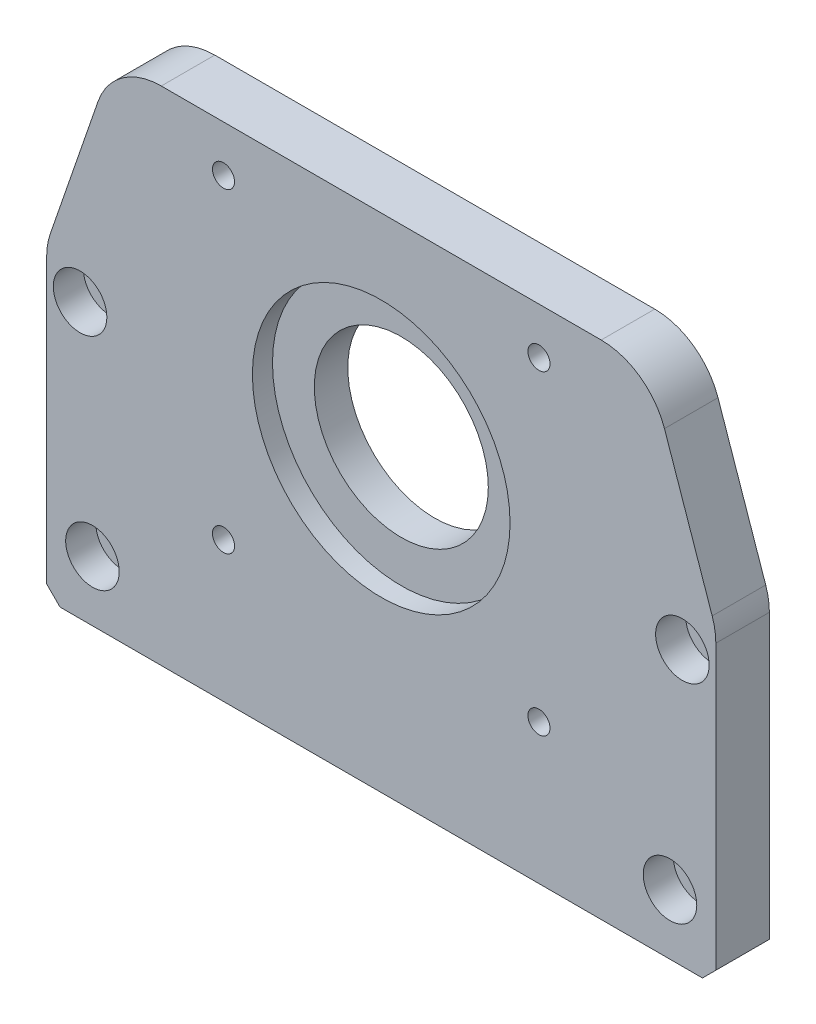
SolidWorks part; units mm, degrees
material "6061铝"
ref_plane "前视基准面" through (0, 0, 0) normal (0, 0, 1) x (1, 0, 0)
ref_plane "上视基准面" through (0, 0, 0) normal (0, 1, 0) x (1, 0, 0)
ref_plane "右视基准面" through (0, 0, 0) normal (1, 0, 0) x (0, 0, -1)
sketch "草图1" plane through (0, 0, 0) normal (0, 0, 1) x (1, 0, 0)
  line L1 (-50, -37.5) -> (50, -37.5)
  line L2 (-50, -37.5) -> (-50, 37.5)
  line L3 (-50, 37.5) -> (50, 37.5)
  line L4 (50, -37.5) -> (50, 37.5)
  line L5 (-50, -37.5) -> (50, 37.5) construction
  line L6 (-50, 37.5) -> (50, -37.5) construction
  point P0 (0, 0)
  dimension "D1" = 100
  dimension "D2" = 75
extrude "凸台-拉伸1" add sketch "草图1" along normal blind 8
sketch "草图3" plane through (0, 0, 0) normal (0, 0, -1) x (-1, 0, 0)
  line L0 (-50, 8.5) -> (-40, 37.5)
  line L1 (-50, -37.5) -> (-50, 37.5) construction
  line L2 (-50, 37.5) -> (50, 37.5) construction
  line L3 (-40, 37.5) -> (-50, 37.5)
  line L4 (-50, 37.5) -> (-50, 8.5)
  line L5 (50, -37.5) -> (-50, -37.5) construction
  line L6 (0, 37.5) -> (0, 59.5078) construction
  line L7 (50, 37.5) -> (50, 8.5)
  line L8 (40, 37.5) -> (50, 37.5)
  line L9 (50, 8.5) -> (40, 37.5)
  dimension "D1" = 46
  dimension "D2" = 10
extrude "切除-拉伸1" cut sketch "草图3" against normal blind 10
fillet "圆角1" radius 10 4 edges at (-50, 8.5, 4) (-40, 37.5, 4) (40, 37.5, 4) (50, 8.5, 4)
chamfer "倒角2" distance 2 angle 45 2 edges at (-50, -37.5, 4) (50, -37.5, 4)
sketch "草图6" plane through (0, 0, 8) normal (0, 0, 1) x (1, 0, 0)
  line L0 (-48, -37.5) -> (48, -37.5) construction
  line L1 (-50, 6.8243) -> (-50, -35.5) construction
  circle A0 centre (0, 7) radius 19.25
  dimension "D1" = 38.5
  dimension "D2" = 44.5
  dimension "D3" = 50
extrude "切除-拉伸2" cut sketch "草图6" against normal blind 3
sketch "草图7" plane through (0, 0, 5) normal (0, 0, 1) x (1, 0, 0)
  circle A0 centre (0, 7) radius 13
  dimension "D1" = 26
extrude "切除-拉伸3" cut sketch "草图7" against normal through all
hole_wizard "打孔尺寸(%根据)内六角圆柱头螺钉的类型1" positions "草图8" profile "草图9" counterbore size "M4" standard "GB" end condition through all
sketch "草图8" plane through (0, 0, 8) normal (0, 0, 1) x (1, 0, 0)
  point P0 (-45, 3.5)
  point P3 (-43.15, -28.5)
  point P6 (43.15, -28.5)
  point P9 (45, 3.5)
sketch "草图9" plane through (-45, 3.5, 8) normal (1, 0, 0) x (0, -1, 0)
  line L0 (0, 0) -> (0, 8)
  line L1 (0, 8) -> (2.2, 8)
  line L3 (2.2, 8) -> (2.2, 4.5)
  line L4 (2.2, 4.5) -> (4, 4.5)
  line L5 (4, 4.5) -> (4, 0)
  line L7 (4, 0) -> (0, 0)
  line L11 (0, -6.35) -> (0, 107.95) construction
  dimension "通孔孔直径" = 4.4
  dimension "通孔孔深度" = 8
  dimension "柱形沉头孔直径" = 8
  dimension "柱形沉头孔深度" = 4.5
hole_wizard "M4 螺纹孔1" positions "草图10" profile "草图12" tap size "M4" standard "GB" end condition through all
sketch "草图10" plane through (0, 0, 8) normal (0, 0, 1) x (1, 0, 0)
  point P0 (-23.57, -16.57)
  point P3 (23.57, -16.57)
  point P6 (23.57, 30.57)
  point P9 (-23.57, 30.57)
sketch "草图12" plane through (-23.57, -16.57, 8) normal (1, 0, 0) x (0, -1, 0)
  line L0 (0, 0) -> (0, 8)
  line L1 (0, 8) -> (1.65, 8)
  line L2 (1.65, 8) -> (1.65, 0)
  line L5 (1.65, 0) -> (0, 0)
  line L11 (0, -6.35) -> (0, 107.95) construction
  dimension "通孔螺纹孔钻头直径" = 3.3
  dimension "通孔螺纹孔钻头深度" = 8
cosmetic thread "孔螺蚊线1" parameters "D2"=4
cosmetic thread "孔螺蚊线2" parameters "D2"=4
cosmetic thread "孔螺蚊线3" parameters "D2"=4
cosmetic thread "孔螺蚊线4" parameters "D2"=4
